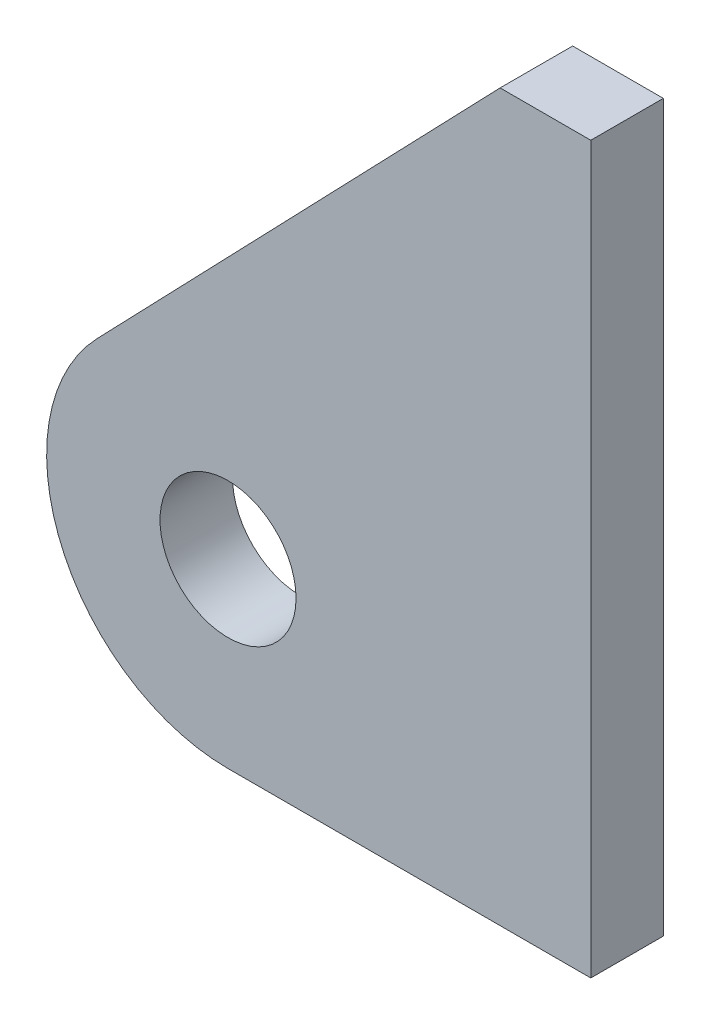
from build123d import *

# Parameters (mm, degrees)
SKETCH1_R           = 7.5
BOSS_EXTRUDE1_DEPTH = 4


with BuildPart() as part:
    # Sketch1 → Boss-Extrude1 (new, symmetric)
    with BuildSketch(Plane.XY):
        with BuildLine():
            Line((0, 0), (0, 80))
            Line((0, 80), (-10, 80))
            Line((-10, 80), (-54.4083313, 33.870832317))
            ThreePointArc((-54.4083313, 33.870832317), (-58.404030079, 12.171099896), (-40, 0))
            Line((-40, 0), (0, 0))
        make_face()
        with Locations((-40, 20)):
            Circle(SKETCH1_R, mode=Mode.SUBTRACT)
    extrude(amount=BOSS_EXTRUDE1_DEPTH, both=True)


solid = part.part
